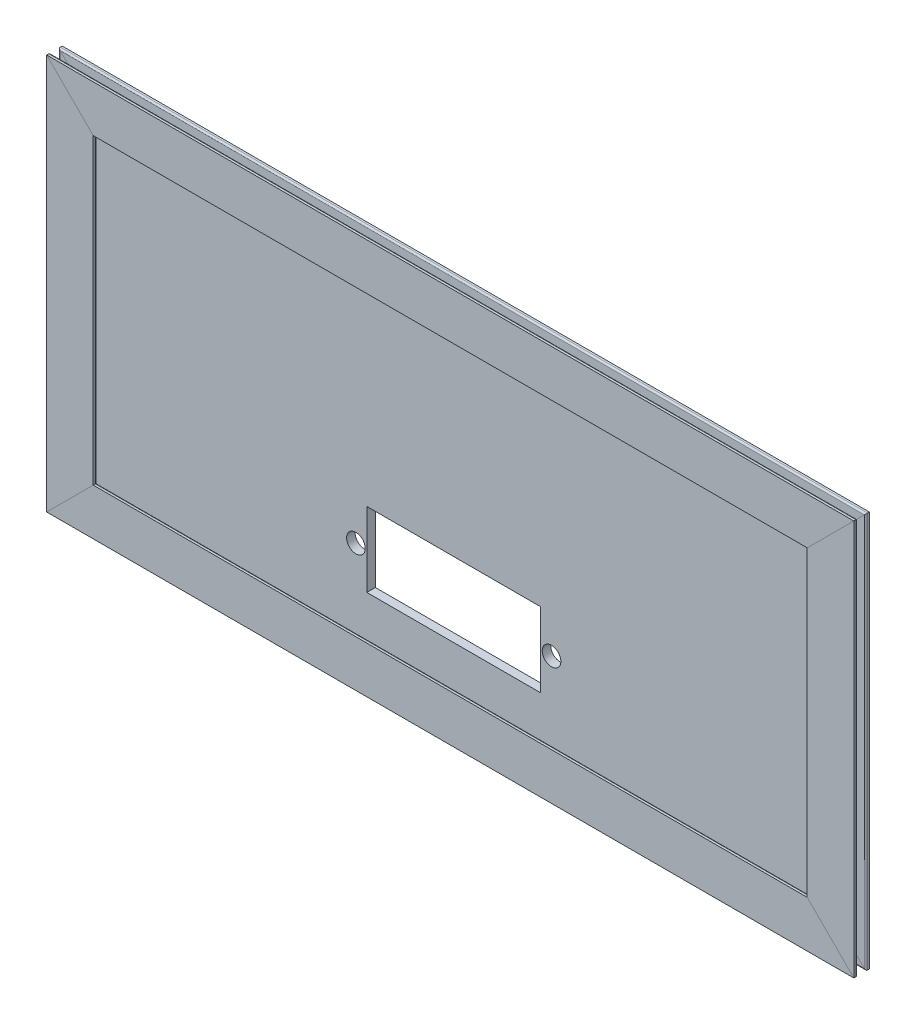
from build123d import *

# Parameters (mm, degrees)
ALUMINIUM_PROFILE_20_X_20_X_2_1_DEPTH      = 506.811388301
ALUMINIUM_PROFILE_20_X_20_X_2_1_DEPTH_BACK = 16.811388301
SKETCH1_W                                  = 6.2
SKETCH1_H                                  = 4.4
SKETCH1_ON_SEGMENT_2_W                     = 6.2
SKETCH1_ON_SEGMENT_2_H                     = 4.4
ALUMINIUM_PROFILE_20_X_20_X_2_1_2_DEPTH    = 258.622776602
SKETCH1_ON_SEGMENT_3_W                     = 6.2
SKETCH1_ON_SEGMENT_3_H                     = 4.4
ALUMINIUM_PROFILE_20_X_20_X_2_1_3_DEPTH    = 523.622776602
SKETCH1_ON_SEGMENT_4_W                     = 6.2
SKETCH1_ON_SEGMENT_4_H                     = 4.4
ALUMINIUM_PROFILE_20_X_20_X_2_1_4_DEPTH    = 258.622776602
SKETCH3_W                                  = 462
SKETCH3_H                                  = 197
BOSS_EXTRUDE1_DEPTH                        = 5.5
SKETCH4_R                                  = 6
SKETCH4_W                                  = 112
SKETCH4_H                                  = 48
CUT_EXTRUDE1_DEPTH                         = 290.683124293


with BuildPart() as part:
    # Sketch1 → Aluminium profile 20 X 20 X 2(1) (new, two sides: drawn at the far end of the back side and taken through both)
    with BuildSketch(Plane(origin=(-245, 112.5, 0), x_dir=(0, 1, 0), z_dir=(1, 0, 0)).offset(-ALUMINIUM_PROFILE_20_X_20_X_2_1_DEPTH_BACK)):
        with BuildLine():
            Line((4.5, 2.75), (14, 2.75))
            ThreePointArc((14, 2.75), (14.707106781, 3.042893219), (15, 3.75))
            Line((15, 3.75), (15, 5))
            Line((15, 5), (-15, 5))
            Line((-15, 5), (-15, 3.75))
            ThreePointArc((-15, 3.75), (-14.707106781, 3.042893219), (-14, 2.75))
            Line((-14, 2.75), (-4.5, 2.75))
            Line((-4.5, 2.75), (-4.5, -2.75))
            Line((-4.5, -2.75), (-14, -2.75))
            ThreePointArc((-14, -2.75), (-14.707106781, -3.042893219), (-15, -3.75))
            Line((-15, -3.75), (-15, -5))
            Line((-15, -5), (15, -5))
            Line((15, -5), (15, -3.75))
            ThreePointArc((15, -3.75), (14.707106781, -3.042893219), (14, -2.75))
            Line((14, -2.75), (4.5, -2.75))
            Line((4.5, -2.75), (4.5, 2.75))
        make_face()
        Rectangle(SKETCH1_W, SKETCH1_H, mode=Mode.SUBTRACT)
    extrude(amount=ALUMINIUM_PROFILE_20_X_20_X_2_1_DEPTH + ALUMINIUM_PROFILE_20_X_20_X_2_1_DEPTH_BACK)

    # Aluminium profile 20 X 20 X 2(1) mitre 1
    split(bisect_by=Plane(origin=(-245, 112.5, 0), x_dir=(-0.707106781, 0.707106781, 0), z_dir=(0.707106781, 0.707106781, 0)), keep=Keep.TOP)

    # Aluminium profile 20 X 20 X 2(1) mitre 2
    split(bisect_by=Plane(origin=(245, 112.5, 0), x_dir=(-0.707106781, -0.707106781, 0), z_dir=(-0.707106781, 0.707106781, 0)), keep=Keep.TOP)


with BuildPart() as body_2:
    # Sketch1 on segment 2 (carried to segment 2) → Aluminium profile 20 X 20 X 2_1 2 (new body)
    with BuildSketch(Plane(origin=(245, 129.311388301, 0), x_dir=(1, 0, 0), z_dir=(0, -1, 0))):
        with BuildLine():
            Line((4.5, 2.75), (14, 2.75))
            ThreePointArc((14, 2.75), (14.707106781, 3.042893219), (15, 3.75))
            Line((15, 3.75), (15, 5))
            Line((15, 5), (-15, 5))
            Line((-15, 5), (-15, 3.75))
            ThreePointArc((-15, 3.75), (-14.707106781, 3.042893219), (-14, 2.75))
            Line((-14, 2.75), (-4.5, 2.75))
            Line((-4.5, 2.75), (-4.5, -2.75))
            Line((-4.5, -2.75), (-14, -2.75))
            ThreePointArc((-14, -2.75), (-14.707106781, -3.042893219), (-15, -3.75))
            Line((-15, -3.75), (-15, -5))
            Line((-15, -5), (15, -5))
            Line((15, -5), (15, -3.75))
            ThreePointArc((15, -3.75), (14.707106781, -3.042893219), (14, -2.75))
            Line((14, -2.75), (4.5, -2.75))
            Line((4.5, -2.75), (4.5, 2.75))
        make_face()
        Rectangle(SKETCH1_ON_SEGMENT_2_W, SKETCH1_ON_SEGMENT_2_H, mode=Mode.SUBTRACT)
    extrude(amount=ALUMINIUM_PROFILE_20_X_20_X_2_1_2_DEPTH)

    # Aluminium profile 20 X 20 X 2_1 2 mitre
    split(bisect_by=Plane(origin=(245, -112.5, 0), x_dir=(-0.707106781, 0.707106781, 0), z_dir=(0.707106781, 0.707106781, 0)), keep=Keep.TOP)

    # Aluminium profile 20 X 20 X 2_1 2 mi 2
    split(bisect_by=Plane(origin=(245, 112.5, 0), x_dir=(0.707106781, 0.707106781, 0), z_dir=(0.707106781, -0.707106781, 0)), keep=Keep.TOP)


with BuildPart() as body_3:
    # Sketch1 on segment 3 (carried to segment 3) → Aluminium profile 20 X 20 X 2_1 3 (new body)
    with BuildSketch(Plane(origin=(261.811388301, -112.5, 0), x_dir=(0, -1, 0), z_dir=(-1, 0, 0))):
        with BuildLine():
            Line((4.5, 2.75), (14, 2.75))
            ThreePointArc((14, 2.75), (14.707106781, 3.042893219), (15, 3.75))
            Line((15, 3.75), (15, 5))
            Line((15, 5), (-15, 5))
            Line((-15, 5), (-15, 3.75))
            ThreePointArc((-15, 3.75), (-14.707106781, 3.042893219), (-14, 2.75))
            Line((-14, 2.75), (-4.5, 2.75))
            Line((-4.5, 2.75), (-4.5, -2.75))
            Line((-4.5, -2.75), (-14, -2.75))
            ThreePointArc((-14, -2.75), (-14.707106781, -3.042893219), (-15, -3.75))
            Line((-15, -3.75), (-15, -5))
            Line((-15, -5), (15, -5))
            Line((15, -5), (15, -3.75))
            ThreePointArc((15, -3.75), (14.707106781, -3.042893219), (14, -2.75))
            Line((14, -2.75), (4.5, -2.75))
            Line((4.5, -2.75), (4.5, 2.75))
        make_face()
        Rectangle(SKETCH1_ON_SEGMENT_3_W, SKETCH1_ON_SEGMENT_3_H, mode=Mode.SUBTRACT)
    extrude(amount=ALUMINIUM_PROFILE_20_X_20_X_2_1_3_DEPTH)

    # Aluminium profile 20 X 20 X 2_1 3 mitre
    split(bisect_by=Plane(origin=(-245, -112.5, 0), x_dir=(0.707106781, 0.707106781, 0), z_dir=(0.707106781, -0.707106781, 0)), keep=Keep.TOP)

    # Aluminium profile 20 X 20 X 2_1 3 mi 2
    split(bisect_by=Plane(origin=(245, -112.5, 0), x_dir=(0.707106781, -0.707106781, 0), z_dir=(-0.707106781, -0.707106781, 0)), keep=Keep.TOP)


with BuildPart() as body_4:
    # Sketch1 on segment 4 (carried to segment 4) → Aluminium profile 20 X 20 X 2_1 4 (new body)
    with BuildSketch(Plane(origin=(-245, -129.311388301, 0), x_dir=(-1, 0, 0), z_dir=(0, 1, 0))):
        with BuildLine():
            Line((4.5, 2.75), (14, 2.75))
            ThreePointArc((14, 2.75), (14.707106781, 3.042893219), (15, 3.75))
            Line((15, 3.75), (15, 5))
            Line((15, 5), (-15, 5))
            Line((-15, 5), (-15, 3.75))
            ThreePointArc((-15, 3.75), (-14.707106781, 3.042893219), (-14, 2.75))
            Line((-14, 2.75), (-4.5, 2.75))
            Line((-4.5, 2.75), (-4.5, -2.75))
            Line((-4.5, -2.75), (-14, -2.75))
            ThreePointArc((-14, -2.75), (-14.707106781, -3.042893219), (-15, -3.75))
            Line((-15, -3.75), (-15, -5))
            Line((-15, -5), (15, -5))
            Line((15, -5), (15, -3.75))
            ThreePointArc((15, -3.75), (14.707106781, -3.042893219), (14, -2.75))
            Line((14, -2.75), (4.5, -2.75))
            Line((4.5, -2.75), (4.5, 2.75))
        make_face()
        Rectangle(SKETCH1_ON_SEGMENT_4_W, SKETCH1_ON_SEGMENT_4_H, mode=Mode.SUBTRACT)
    extrude(amount=ALUMINIUM_PROFILE_20_X_20_X_2_1_4_DEPTH)

    # Aluminium profile 20 X 20 X 2_1 4 mitre
    split(bisect_by=Plane(origin=(-245, -112.5, 0), x_dir=(-0.707106781, -0.707106781, 0), z_dir=(-0.707106781, 0.707106781, 0)), keep=Keep.TOP)

    # Aluminium profile 20 X 20 X 2_1 4 mi 2
    split(bisect_by=Plane(origin=(-245, 112.5, 0), x_dir=(0.707106781, -0.707106781, 0), z_dir=(-0.707106781, -0.707106781, 0)), keep=Keep.TOP)


with BuildPart() as body_5:
    # Sketch3 → Boss-Extrude1 (new body)
    with BuildSketch(Plane.XY.offset(-2.75)):
        Rectangle(SKETCH3_W, SKETCH3_H)
    extrude(amount=BOSS_EXTRUDE1_DEPTH)

    # Sketch4 → Cut-Extrude1 (cut, through all)
    with BuildSketch(Plane(origin=(0, 0, -2.75), x_dir=(-1, 0, 0), z_dir=(0, 0, -1))):
        with Locations((-63, -47.5)):
            Circle(SKETCH4_R)
        with Locations((63, -47.5)):
            Circle(SKETCH4_R)
        with Locations((0, -47.5)):
            Rectangle(SKETCH4_W, SKETCH4_H)
    extrude(amount=-CUT_EXTRUDE1_DEPTH, mode=Mode.SUBTRACT)


solid = Compound([part.part, body_2.part, body_3.part, body_4.part, body_5.part])
